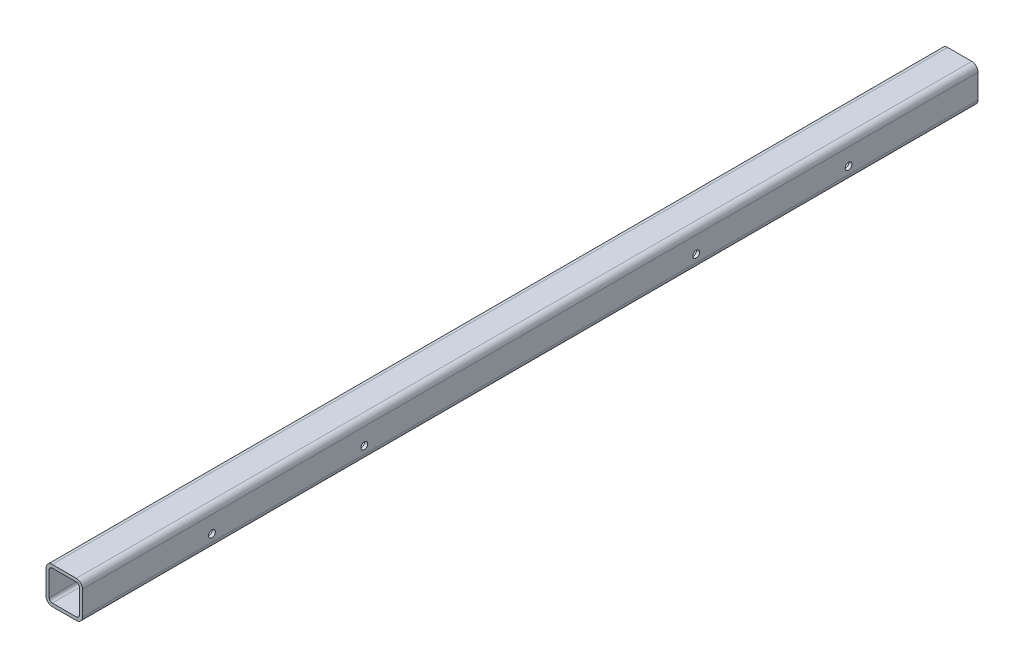
from build123d import *

# Parameters (mm, degrees)
BOSS_EXTRUDE1_DEPTH = 1716
SKETCH2_R           = 6.5
CUT_EXTRUDE1_DEPTH  = 1719.853105998
LPATTERN1_COUNT     = 2
LPATTERN1_PITCH     = 928


with BuildPart() as part:
    # Sketch1 → Boss-Extrude1 (new body)
    with BuildSketch(Plane.XY):
        with BuildLine():
            Line((12, 0), (58, 0))
            ThreePointArc((58, 0), (66.485281374, 3.514718626), (70, 12))
            Line((70, 12), (70, 58))
            ThreePointArc((70, 58), (66.485281374, 66.485281374), (58, 70))
            Line((58, 70), (12, 70))
            ThreePointArc((12, 70), (3.514718626, 66.485281374), (0, 58))
            Line((0, 58), (0, 12))
            ThreePointArc((0, 12), (3.514718626, 3.514718626), (12, 0))
        make_face()
        with BuildLine():
            Line((12, 6), (58, 6))
            ThreePointArc((58, 6), (62.242640687, 7.757359313), (64, 12))
            Line((64, 12), (64, 58))
            ThreePointArc((64, 58), (62.242640687, 62.242640687), (58, 64))
            Line((58, 64), (12, 64))
            ThreePointArc((12, 64), (7.757359313, 62.242640687), (6, 58))
            Line((6, 58), (6, 12))
            ThreePointArc((6, 12), (7.757359313, 7.757359313), (12, 6))
        make_face(mode=Mode.SUBTRACT)
    extrude(amount=BOSS_EXTRUDE1_DEPTH)

    # Sketch2 → Cut-Extrude1 (cut, through all)
    with BuildSketch(Plane.ZY):
        with Locations((248, 26)):
            Circle(SKETCH2_R)
        with Locations((540, 26)):
            Circle(SKETCH2_R)
    cut_extrude1 = extrude(amount=-CUT_EXTRUDE1_DEPTH, mode=Mode.SUBTRACT)

    # LPattern1: Cut-Extrude1 ×2
    with Locations(*[(0, 0, i * LPATTERN1_PITCH) for i in range(1, LPATTERN1_COUNT)]):
        add(cut_extrude1, mode=Mode.SUBTRACT)


solid = part.part
